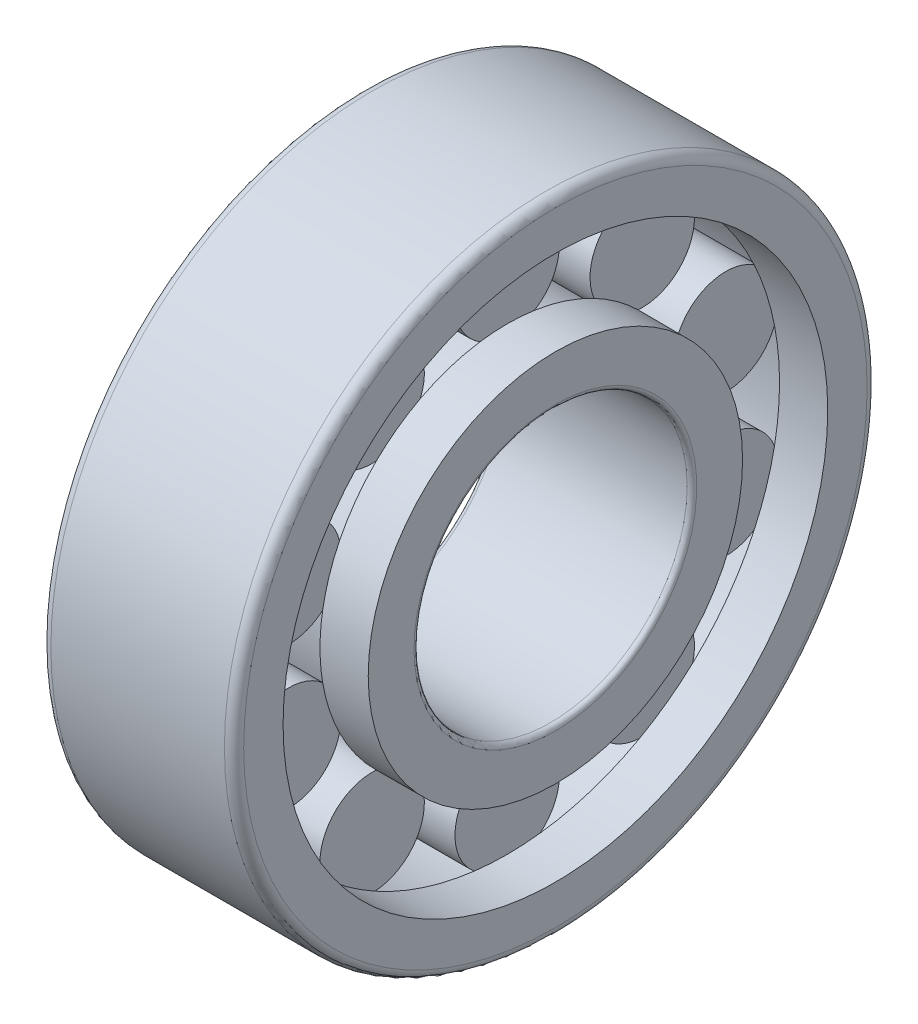
SolidWorks part; units mm, degrees
revolve "基体-旋转" add sketch "草图2" angle 360 about L0
sketch "草图2" plane through (0, 0, 0) normal (0, 0, 1) x (1, 0, 0)
  line L0 (-10.0801, 0) -> (21.9267, 0) construction
  line L1 (3, 11.05) -> (9, 11.05)
  line L2 (0, 11.65) -> (3, 11.65)
  line L3 (0, 11.65) -> (0, 8.8)
  line L4 (0.3, 8.5) -> (11.7, 8.5)
  line L5 (12, 11.65) -> (12, 8.8)
  line L6 (3, 11.05) -> (3, 11.65)
  line L7 (9, 11.05) -> (9, 11.65)
  line L8 (9, 11.65) -> (12, 11.65)
  arc A0 (11.7, 8.5) -> (12, 8.8) centre (11.7, 8.8) ccw
  arc A1 (0, 8.8) -> (0.3, 8.5) centre (0.3, 8.8) ccw
  point P13 (12, 8.5)
  point P16 (0, 8.5)
ref_plane "基准面1" through (0, 0, 0) normal (0, 0, 1) x (1, 0, 0)
ref_plane "基准面2" through (0, 0, 0) normal (0, 1, 0) x (1, 0, 0)
ref_plane "基准面3" through (0, 0, 0) normal (1, 0, 0) x (0, 0, -1)
sketch "尺寸草图" plane through (0, 0, 0) normal (0, 0, 1) x (1, 0, 0)
  line L0 (0, 0) -> (0.3, 0)
  line L1 (0.3, 0) -> (0.9, 0)
  line L2 (0.9, 0) -> (12.9, 0)
  line L3 (12.9, 0) -> (29.9, 0)
  line L4 (29.9, 0) -> (52, 0)
  line L5 (52, 0) -> (92, 0)
  line L7 (92, 0) -> (127.1, 0)
sketch "草图3" plane through (0, 0, 0) normal (0, 0, 1) x (1, 0, 0)
  line L0 (9, 11.65) -> (9, -11.65) construction
  line L2 (-1.6039, 14.3) -> (13.5036, 14.3) construction
  line L4 (3, 14.3) -> (9, 14.3)
  line L5 (3, 14.3) -> (3, 11.0499)
  line L6 (3, 11.0499) -> (9, 11.0499)
  line L7 (9, 14.3) -> (9, 11.0499)
  line L8 (3, -11.65) -> (3, 11.65) construction
revolve "凸台-旋转1" add sketch "草图3" angle 360 about L2
sketch "草图4" plane through (0, 0, 0) normal (0, 0, 1) x (1, 0, 0)
  line L0 (0, 0) -> (17.8006, 0) construction
  line L1 (-10.0801, 0) -> (21.9267, 0) construction
  line L2 (9, 16.95) -> (12, 16.95)
  line L3 (0.6, 20) -> (11.4, 20)
  line L4 (0, 19.4) -> (0, 16.95)
  line L5 (0, 16.95) -> (3, 16.95)
  line L6 (12, 19.4) -> (12, 16.95)
  line L7 (3, 17.55) -> (9, 17.55)
  line L8 (3, 17.55) -> (3, 16.95)
  line L10 (9, 17.55) -> (9, 16.95)
  arc A0 (11.4, 20) -> (12, 19.4) centre (11.4, 19.4) cw
  arc A1 (0.6, 20) -> (0, 19.4) centre (0.6, 19.4) ccw
  point P15 (12, 20)
  point P18 (0, 20)
revolve "凸台-旋转2" add sketch "草图4" angle 360 about L0
pattern_circular "阵列(圆周)1" count 10 over 360 about axis through (0, 0, 0) along (1, 0, 0) of "凸台-旋转1"
equation "\"DD@草图2\" = \"内径@尺寸草图\""
equation "\"FW@草图2\" = \"参考FW@尺寸草图\""
equation "\"D1@草图2\" = \"倒角小@尺寸草图\""
equation "\"EW@草图4\" = \"参考EW@尺寸草图\""
equation "\"D@草图4\" = \"外径@尺寸草图\""
equation "\"D2@草图4\" = \"倒角大@尺寸草图\""
equation "\"B@草图4\" = \"宽度@尺寸草图\""
equation "\"D2@草图2\" = \"B@草图4\""
equation "\"滚珠位置@草图2\" = \"D2@草图2\"/4"
equation "\"D3@草图4\" = \"D2@草图4\""
equation "\"D1@草图3\" =  ( \"EW@草图4\" - \"FW@草图2\" )  / 4 + \"FW@草图2\" / 2"
equation "\"D2@草图3\" =  0.25*( \"EW@草图4\" - \"FW@草图2\" ) +0.0001"
equation "\"D4@草图2\" = \"FW@草图2\" + 4 *\"D1@草图2\""
equation "\"D1@阵列(圆周)1\" =0.75* \"D1@草图3\" * 3.14 / \"D2@草图3\""
